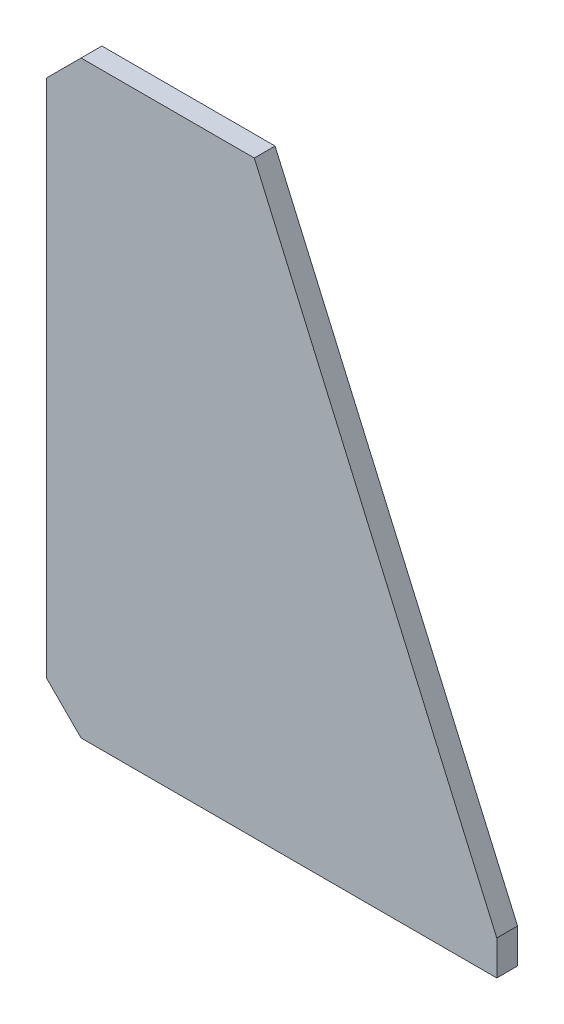
from build123d import *

# Parameters (mm, degrees)
BOSS_EXTRUDE1_DEPTH = 3
CHAMFER1_SIZE       = 10


with BuildPart() as part:
    # Sketch1 → Boss-Extrude1 (new, symmetric)
    with BuildSketch(Plane.XY):
        Polygon((0, 170), (0, 0), (130, 0), (130, 10), (60, 170), align=None)
    extrude(amount=BOSS_EXTRUDE1_DEPTH, both=True)

    # Chamfer1
    chamfer1_edges = [part.edges().sort_by_distance(p)[0] for p in [
        (0, 0, 0),
        (0, 170, 0),
    ]]
    chamfer(chamfer1_edges, length=CHAMFER1_SIZE)


solid = part.part
